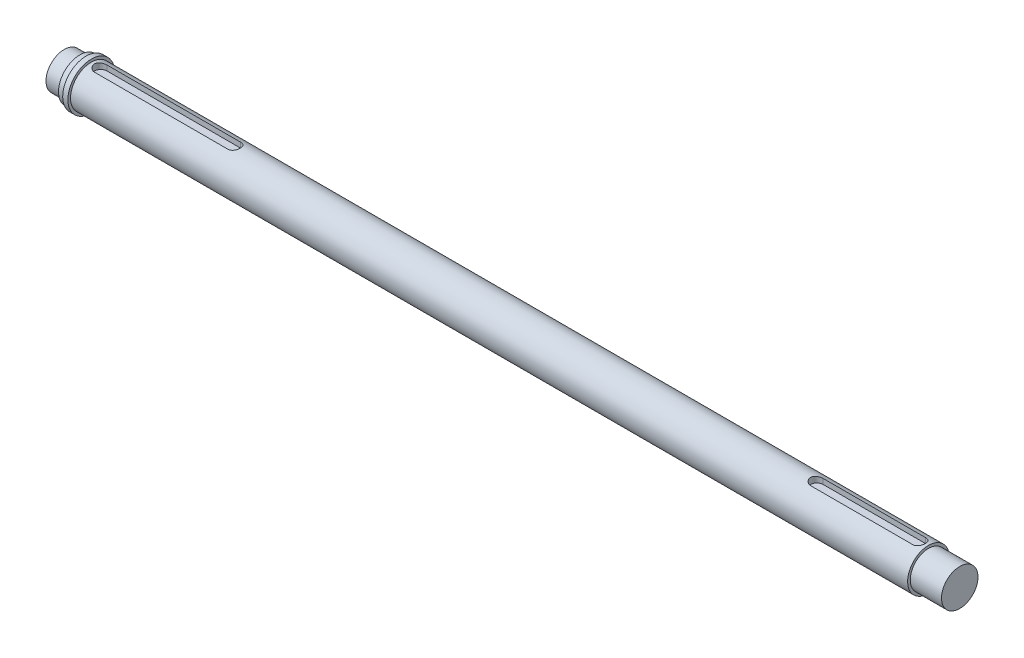
SolidWorks part; units mm, degrees
ref_plane "前视基准面" through (0, 0, 0) normal (0, 0, 1) x (1, 0, 0)
ref_plane "上视基准面" through (0, 0, 0) normal (0, 1, 0) x (1, 0, 0)
ref_plane "右视基准面" through (0, 0, 0) normal (1, 0, 0) x (0, 0, -1)
sketch "草图1" plane through (0, 0, 0) normal (1, 0, 0) x (0, 0, -1)
  circle A0 centre (0, 0) radius 20
extrude "凸台-拉伸1" add sketch "草图1" along normal blind 803
sketch "草图2" plane through (803, 0, 0) normal (1, 0, 0) x (0, 0, -1)
  circle A0 centre (0, 0) radius 17.5
extrude "凸台-拉伸2" add sketch "草图2" along normal blind 30
sketch "草图3" plane through (0, 0, 0) normal (-1, 0, 0) x (0, 0, 1)
  circle A0 centre (0, 0) radius 22.5
extrude "凸台-拉伸3" add sketch "草图3" along normal blind 5
sketch "草图4" plane through (-5, 0, 0) normal (-1, 0, 0) x (0, 0, 1)
  circle A0 centre (0, 0) radius 20.5
extrude "凸台-拉伸4" add sketch "草图4" along normal blind 6
sketch "草图5" plane through (-11, 0, 0) normal (-1, 0, 0) x (0, 0, 1)
  circle A0 centre (0, 0) radius 17.5
extrude "凸台-拉伸5" add sketch "草图5" along normal blind 15
ref_plane "基准面1" through (0, 20, 0) normal (0, 1, 0) x (1, 0, 0)
sketch "草图6" plane through (0, 20, 0) normal (0, 1, 0) x (1, 0, 0)
  line L0 (9, 0) -> (137, 0) construction
  line L1 (0, -20) -> (0, 20) construction
  line L2 (9, 6) -> (137, 6)
  line L3 (9, -6) -> (137, -6)
  line L4 (794, 0) -> (696, 0) construction
  line L5 (803, -17.5) -> (803, 17.5) construction
  line L6 (794, -6) -> (696, -6)
  line L7 (794, 6) -> (696, 6)
  arc A0 (9, 6) -> (9, -6) centre (9, 0) ccw
  arc A1 (137, -6) -> (137, 6) centre (137, 0) ccw
  arc A2 (794, -6) -> (794, 6) centre (794, 0) ccw
  arc A3 (696, 6) -> (696, -6) centre (696, 0) ccw
  point P5 (73, 0)
  point P14 (745, 0)
  dimension "D1" = 128
  dimension "D2" = 9
  dimension "D3" = 9
  dimension "D4" = 98
extrude "切除-拉伸1" cut sketch "草图6" against normal blind 5.92
